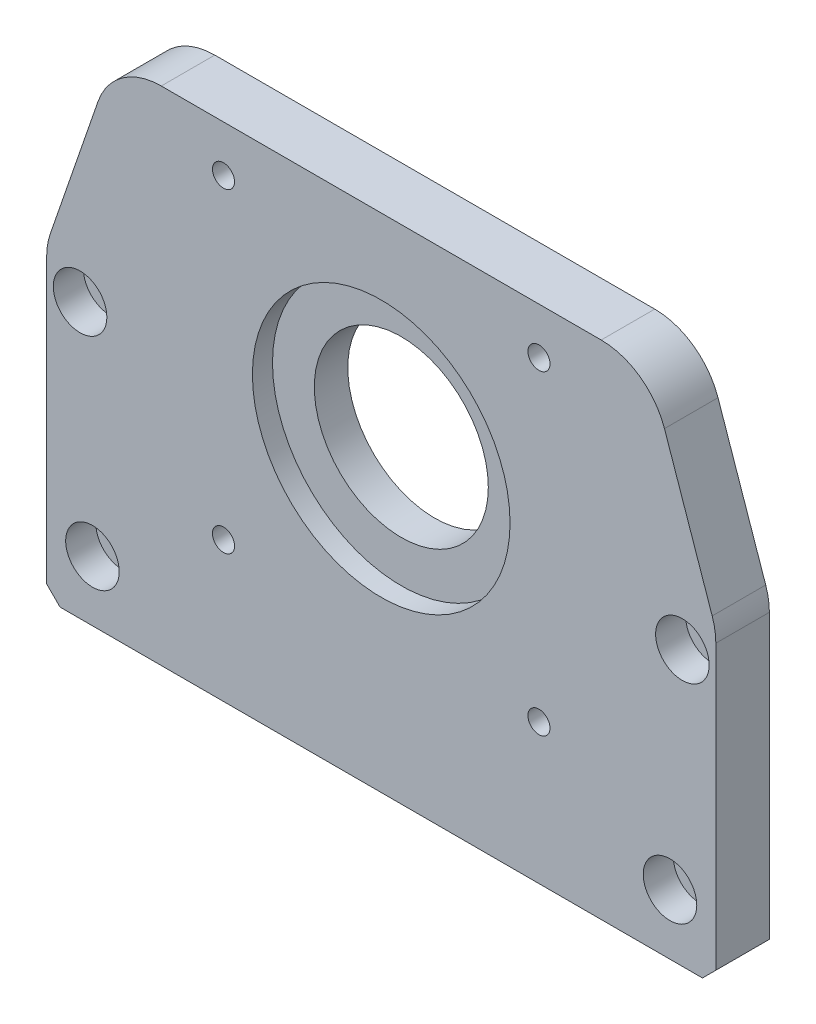
from build123d import *

# Parameters (mm, degrees)
SKETCH_1_W                = 100
SKETCH_1_H                = 75
EXTRUDE_1_DEPTH           = 8
CUT_EXTRUDE_1_DEPTH       = 10
FILLET_1_R                = 10
CHAMFER_2_SIZE            = 2
SKETCH_6_R                = 19.25
CUT_EXTRUDE_2_DEPTH       = 3
SKETCH_7_R                = 13
CUT_EXTRUDE_3_DEPTH       = 63.69968102
HOLE_WIZARD_1_D           = 4.4
HOLE_WIZARD_1_CBORE_D     = 8
HOLE_WIZARD_1_CBORE_DEPTH = 4.5
HOLE_WIZARD_M4_1_D        = 3.3


with BuildPart() as part:
    # 草图1 → 凸台-拉伸1 (new body)
    with BuildSketch(Plane.XY):
        Rectangle(SKETCH_1_W, SKETCH_1_H)
    extrude(amount=EXTRUDE_1_DEPTH)

    # 草图3 → 切除-拉伸1 (cut)
    with BuildSketch(Plane(origin=(0, 0, 0), x_dir=(-1, 0, 0), z_dir=(0, 0, -1))):
        Polygon((-50, 8.5), (-40, 37.5), (-50, 37.5), align=None)
        Polygon((50, 37.5), (50, 8.5), (40, 37.5), align=None)
    extrude(amount=-CUT_EXTRUDE_1_DEPTH, mode=Mode.SUBTRACT)

    # 圆角1
    fillet_1_edges = [part.edges().sort_by_distance(p)[0] for p in [
        (50, 8.5, 4),
        (40, 37.5, 4),
        (-40, 37.5, 4),
        (-50, 8.5, 4),
    ]]
    fillet(fillet_1_edges, radius=FILLET_1_R)

    # 倒角2
    chamfer_2_edges = [part.edges().sort_by_distance(p)[0] for p in [
        (50, -37.5, 4),
        (-50, -37.5, 4),
    ]]
    chamfer(chamfer_2_edges, length=CHAMFER_2_SIZE)

    # 草图6 → 切除-拉伸2 (cut)
    with BuildSketch(Plane.XY.offset(8)):
        with Locations((0, 7)):
            Circle(SKETCH_6_R)
    extrude(amount=-CUT_EXTRUDE_2_DEPTH, mode=Mode.SUBTRACT)

    # 草图7 → 切除-拉伸3 (cut, through all)
    with BuildSketch(Plane.XY.offset(5)):
        with Locations((0, 7)):
            Circle(SKETCH_7_R)
    extrude(amount=-CUT_EXTRUDE_3_DEPTH, mode=Mode.SUBTRACT)

    # 打孔尺寸(%根据)内六角圆柱头螺钉的类型1 (through all)
    with Locations(Plane.XY.offset(8)):
        with Locations((-45, 3.5), (-43.15, -28.5), (43.15, -28.5), (45, 3.5)):
            CounterBoreHole(HOLE_WIZARD_1_D / 2, HOLE_WIZARD_1_CBORE_D / 2, HOLE_WIZARD_1_CBORE_DEPTH)

    # M4 螺纹孔1 (through all)
    with Locations(Plane.XY.offset(8)):
        with Locations((-23.57, -16.57), (23.57, -16.57), (23.57, 30.57), (-23.57, 30.57)):
            Hole(HOLE_WIZARD_M4_1_D / 2)


solid = part.part
